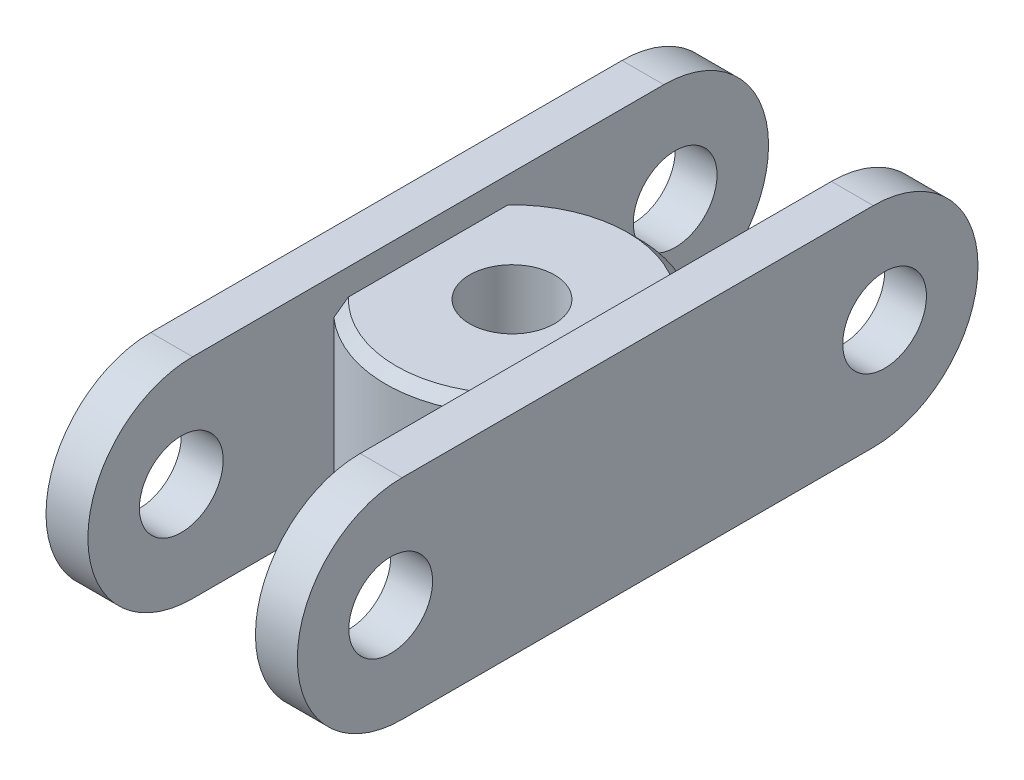
SolidWorks part; units mm, degrees
ref_plane "Plan de face" through (0, 0, 0) normal (0, 0, 1) x (1, 0, 0)
ref_plane "Plan de dessus" through (0, 0, 0) normal (0, 1, 0) x (1, 0, 0)
ref_plane "Plan de droite" through (0, 0, 0) normal (1, 0, 0) x (0, 0, -1)
sketch "Sketch1" plane through (0, 0, 0) normal (0, 1, 0) x (1, 0, 0)
  circle A0 centre (0, 0) radius 4.05
  circle A1 centre (0, 0) radius 12.05
  dimension "D1" = 8.1
  dimension "D2" = 8
extrude "Boss.-Extru.1" add sketch "Sketch1" along normal blind 15
chamfer "Chamfer1" distance 1 angle 45 1 edges at (0, 15, 12.05)
ref_plane "Plan1" through (12, 0, 0) normal (1, 0, 0) x (0, 0, -1)
sketch "Sketch5" plane through (0, 15, 0) normal (0, 1, 0) x (1, 0, 0)
  line L1 (15, 18.778) -> (8, 18.778)
  line L2 (15, 18.778) -> (15, -22.1025)
  line L3 (15, -22.1025) -> (8, -22.1025)
  line L4 (8, 18.778) -> (8, -22.1025)
  line L5 (0, 28.6852) -> (0, -31.0712) construction
  line L6 (-8, 18.778) -> (-8, -22.1025)
  line L7 (-15, -22.1025) -> (-8, -22.1025)
  line L8 (-15, 18.778) -> (-15, -22.1025)
  line L9 (-15, 18.778) -> (-8, 18.778)
  dimension "D1" = 8
  dimension "D2" = 8
extrude "Cut-Extrude1" cut sketch "Sketch5" against normal up to next contours L6 L7 L8 L9 | L4 L3 L2 L1
sketch "Sketch6" plane through (8, 0, 0) normal (1, 0, 0) x (0, 0, -1)
  line L0 (0, 15) -> (0, 0) construction
  line L1 (7.6225, 15) -> (-7.6225, 15) construction
  line L2 (-23.5799, 7.5) -> (23.5799, 7.5) construction
  line L3 (22.5, 7.5) -> (-22.5, 7.5) construction
  line L4 (22.5, -2.5) -> (-22.5, -2.5)
  line L5 (22.5, 17.5) -> (-22.5, 17.5)
  arc A0 (22.5, -2.5) -> (22.5, 17.5) centre (22.5, 7.5) ccw
  arc A1 (-22.5, 17.5) -> (-22.5, -2.5) centre (-22.5, 7.5) ccw
  circle A2 centre (23.5799, 7.5) radius 4
  circle A3 centre (-23.5799, 7.5) radius 4
  point P8 (0, 7.5)
  dimension "D1" = 8
extrude "Boss.-Extru.4" add sketch "Sketch6" along normal blind 4
mirror "Mirror1" about plane through (0, 0, 0) normal (1, 0, 0) of "Boss.-Extru.4"
